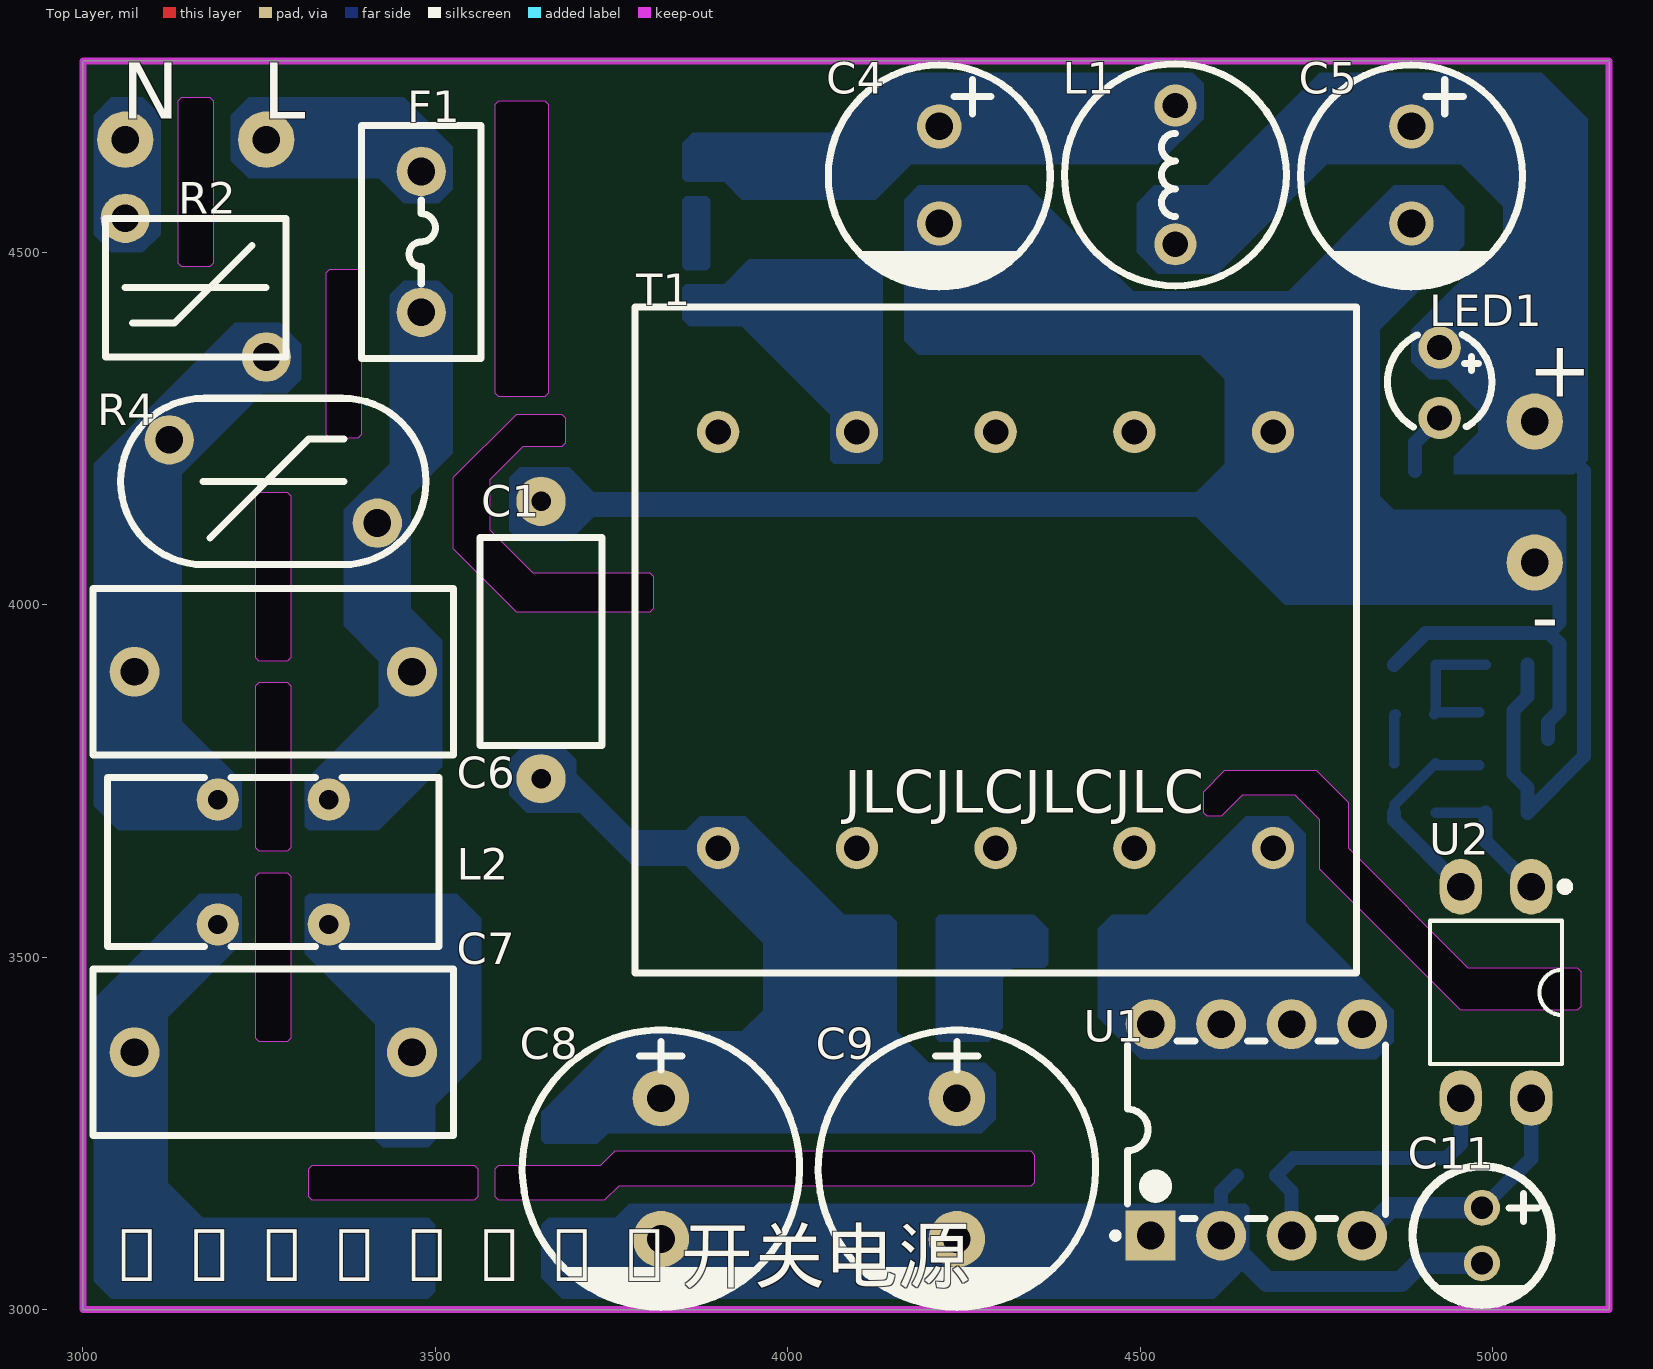
[diagram p0: Top Layer view]
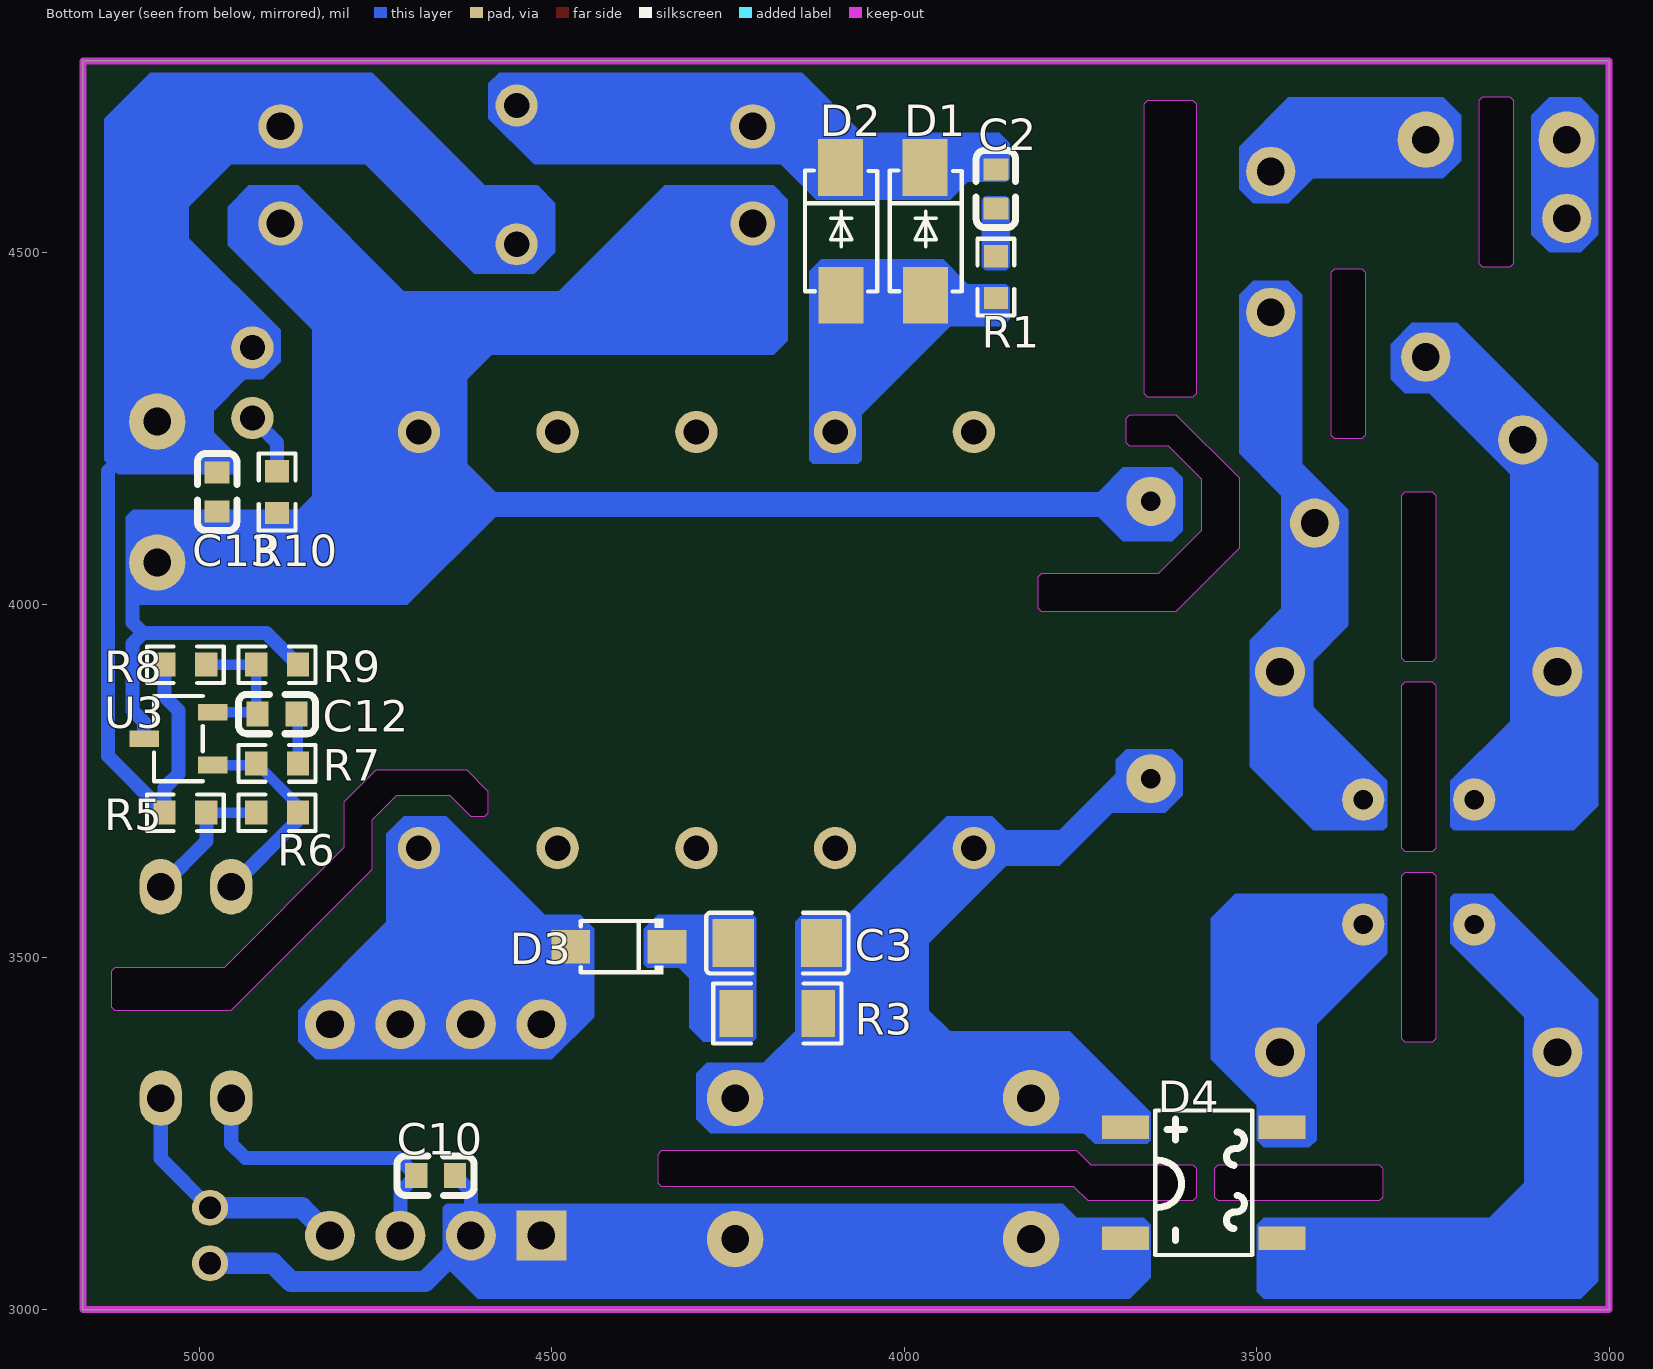
[diagram p1: Bottom Layer view, seen from below]
# Altium PCB MISC51479.pcbdoc
Units mil, origin at the board's own origin, x right, y up, seen from the top; angles counter-clockwise.
Board outline 2165.35 x 1771.65 mil, 2 copper layers (Top Layer, Bottom Layer), stack 62.206 mil thick; 35 components, 22 nets, 95 pads, 0 vias.

## Layer stack, top to bottom
Top Solder Mask Layer: solder mask 0.394, Dk 3.3
Top Layer: signal copper 1.379
Dielectric1: surface 59.449, FR4, Dk 4.5
Bottom Layer: signal copper 1.378
Bottom Solder Mask Layer: solder mask 0.394, Dk 3.3

## Board outline
3000,4771.65 3000,3000 5165.35,3000 5165.35,4771.65
cut-out: 3135,4715 3140,4720 3180,4720 3185,4715 3185,4485 3180,4480 3140,4480 3135,4485
cut-out: 3345,4471.26 3350,4476.26 3390,4476.26 3395,4471.26 3395,4241.26 3390,4236.26 3350,4236.26 3345,4241.26
cut-out: 3245,3885 3250,3890 3290,3890 3295,3885 3295,3655 3290,3650 3250,3650 3245,3655
cut-out: 3245,3615 3250,3620 3290,3620 3295,3615 3295,3385 3290,3380 3250,3380 3245,3385
cut-out: 3325,3155 3320,3160 3320,3200 3325,3205 3555,3205 3560,3200 3560,3160 3555,3155
cut-out: 3585,3200 3590,3205 3735,3205 3755,3225 4345,3225 4350,3220 4350,3180 4345,3175 3760,3175 3740,3155 3590,3155 3585,3160
cut-out: 3680,4225 3685,4230 3685,4265 3680,4270 3615,4270 3525,4180 3525,4080 3615,3990 3805,3990 3810,3995 3810,4040 3805,4045 3638.62,4045 3577.95,4105.67 3577.95,4177.95 3625,4225
cut-out: 3585,4710 3590,4715 3655,4715 3660,4710 3660,4300 3655,4295 3590,4295 3585,4300
cut-out: 4795,3720 4795,3655 4965,3485 5120,3485 5125,3480 5125,3430 5120,3425 4955,3425 4755,3625 4755,3695 4720,3730 4645,3730 4615,3700 4595,3700 4590,3705 4590,3735 4620,3765 4750,3765
cut-out: 3245,4155 3250,4160 3290,4160 3295,4155 3295,3925 3290,3920 3250,3920 3245,3925

## Design rules (kind name [scope] priority, off if disabled: settings)
BoardOutlineClearance copperThickness2oz_1 [All] p2 off: genericclearance=7.99 ignorepadtopadclearanceinfootprint=FALSE except(0: Arc-SplitContinuation Track-SplitContinuation SMDPad-SplitContinuation THPad-SplitContinuation Via-SplitContinuation Fill-SplitContinuation Region-SplitContinuation Poly-SplitContinuation Text-SplitContinuation Hole-SplitContinuation; 5.98: Arc-CutoutEdge Track-CutoutEdge SMDPad-CutoutEdge THPad-CutoutEdge Via-CutoutEdge Text-CutoutEdge; 6.9: Hole-OutlineEdge Hole-CutoutEdge; 10: Poly-OutlineEdge Poly-CutoutEdge; 11.81: Arc-OutlineEdge Track-OutlineEdge SMDPad-OutlineEdge THPad-OutlineEdge Via-OutlineEdge Fill-OutlineEdge Region-OutlineEdge Text-OutlineEdge Fill-CutoutEdge Region-CutoutEdge)
BoardOutlineClearance Plane_innerPlane_1 [All] p4 off: genericclearance=4.02 ignorepadtopadclearanceinfootprint=FALSE except(0: Arc-SplitContinuation Track-SplitContinuation SMDPad-SplitContinuation THPad-SplitContinuation Via-SplitContinuation Fill-SplitContinuation Region-SplitContinuation Poly-SplitContinuation Text-SplitContinuation Hole-SplitContinuation; 5.98: Arc-CutoutEdge Track-CutoutEdge SMDPad-CutoutEdge THPad-CutoutEdge Via-CutoutEdge Text-CutoutEdge; 6.9: Hole-OutlineEdge Hole-CutoutEdge; 10: Poly-OutlineEdge Poly-CutoutEdge; 11.81: Arc-OutlineEdge Track-OutlineEdge SMDPad-OutlineEdge THPad-OutlineEdge Via-OutlineEdge Fill-OutlineEdge Region-OutlineEdge Text-OutlineEdge Fill-CutoutEdge Region-CutoutEdge)
BoardOutlineClearance Copper_copperRegion_1 [All] p6 off: genericclearance=4.02 ignorepadtopadclearanceinfootprint=FALSE except(0: Arc-SplitContinuation Track-SplitContinuation SMDPad-SplitContinuation THPad-SplitContinuation Via-SplitContinuation Fill-SplitContinuation Region-SplitContinuation Poly-SplitContinuation Text-SplitContinuation Hole-SplitContinuation; 5.98: Arc-CutoutEdge Track-CutoutEdge SMDPad-CutoutEdge THPad-CutoutEdge Via-CutoutEdge Text-CutoutEdge; 6.9: Hole-OutlineEdge Hole-CutoutEdge; 10: Poly-OutlineEdge Poly-CutoutEdge; 11.81: Arc-OutlineEdge Track-OutlineEdge SMDPad-OutlineEdge THPad-OutlineEdge Via-OutlineEdge Fill-OutlineEdge Region-OutlineEdge Text-OutlineEdge Fill-CutoutEdge Region-CutoutEdge)
BoardOutlineClearance copperThickness1oz_1 [All] p8: genericclearance=4.02 ignorepadtopadclearanceinfootprint=FALSE except(0: Arc-SplitContinuation Track-SplitContinuation SMDPad-SplitContinuation THPad-SplitContinuation Via-SplitContinuation Fill-SplitContinuation Region-SplitContinuation Poly-SplitContinuation Text-SplitContinuation Hole-SplitContinuation; 5.98: Arc-CutoutEdge Track-CutoutEdge SMDPad-CutoutEdge THPad-CutoutEdge Via-CutoutEdge Text-CutoutEdge; 6.9: Hole-OutlineEdge Hole-CutoutEdge; 10: Poly-OutlineEdge Poly-CutoutEdge; 11.81: Arc-OutlineEdge Track-OutlineEdge SMDPad-OutlineEdge THPad-OutlineEdge Via-OutlineEdge Fill-OutlineEdge Region-OutlineEdge Text-OutlineEdge Fill-CutoutEdge Region-CutoutEdge)
Clearance copperThickness2oz [All] p1 off: gap=7.99 ignorepadtopadclearanceinfootprint=FALSE except(5.98: SMDPad-Track SMDPad-SMDPad THPad-Track SMDPad-THPad THPad-THPad Track-Via SMDPad-Via THPad-Via Via-Via Fill-SMDPad Region-SMDPad Fill-THPad Region-THPad Fill-Via Region-Via Fill-Fill Fill-Region Region-Region Arc-Track Arc-SMDPad Arc-THPad Arc-Via Fill-Arc Region-Arc Arc-Arc Text-Track SMDPad-Text Text-THPad Text-Via Fill-Text Region-Text Arc-Text Text-Text; 6.9: Hole-Track Hole-SMDPad Hole-THPad Hole-Via Fill-Hole Region-Hole Hole-Arc Hole-Text; 10: Poly-Track Poly-SMDPad Poly-THPad Poly-Via Poly-Fill Poly-Region Poly-Poly Poly-Arc Poly-Text Poly-Hole; 11.81: Fill-Track Region-Track)
Clearance Plane_innerPlane [All] p3 off: gap=4.02 ignorepadtopadclearanceinfootprint=FALSE except(5.98: SMDPad-Track SMDPad-SMDPad THPad-Track SMDPad-THPad THPad-THPad Track-Via SMDPad-Via THPad-Via Via-Via Fill-SMDPad Region-SMDPad Fill-THPad Region-THPad Fill-Via Region-Via Fill-Fill Fill-Region Region-Region Arc-Track Arc-SMDPad Arc-THPad Arc-Via Fill-Arc Region-Arc Arc-Arc Text-Track SMDPad-Text Text-THPad Text-Via Fill-Text Region-Text Arc-Text Text-Text; 6.9: Hole-Track Hole-SMDPad Hole-THPad Hole-Via Fill-Hole Region-Hole Hole-Arc Hole-Text; 10: Poly-Track Poly-SMDPad Poly-THPad Poly-Via Poly-Fill Poly-Region Poly-Poly Poly-Arc Poly-Text Poly-Hole; 11.81: Fill-Track Region-Track)
Clearance Copper_copperRegion [All] p5 off: gap=4.02 ignorepadtopadclearanceinfootprint=FALSE except(5.98: SMDPad-Track SMDPad-SMDPad THPad-Track SMDPad-THPad THPad-THPad Track-Via SMDPad-Via THPad-Via Via-Via Fill-SMDPad Region-SMDPad Fill-THPad Region-THPad Fill-Via Region-Via Fill-Fill Fill-Region Region-Region Arc-Track Arc-SMDPad Arc-THPad Arc-Via Fill-Arc Region-Arc Arc-Arc Text-Track SMDPad-Text Text-THPad Text-Via Fill-Text Region-Text Arc-Text Text-Text; 6.9: Hole-Track Hole-SMDPad Hole-THPad Hole-Via Fill-Hole Region-Hole Hole-Arc Hole-Text; 10: Poly-Track Poly-SMDPad Poly-THPad Poly-Via Poly-Fill Poly-Region Poly-Poly Poly-Arc Poly-Text Poly-Hole; 11.81: Fill-Track Region-Track)
Clearance copperThickness1oz [All] p7: gap=4.02 ignorepadtopadclearanceinfootprint=FALSE except(5.98: SMDPad-Track SMDPad-SMDPad THPad-Track SMDPad-THPad THPad-THPad Track-Via SMDPad-Via THPad-Via Via-Via Fill-SMDPad Region-SMDPad Fill-THPad Region-THPad Fill-Via Region-Via Fill-Fill Fill-Region Region-Region Arc-Track Arc-SMDPad Arc-THPad Arc-Via Fill-Arc Region-Arc Arc-Arc Text-Track SMDPad-Text Text-THPad Text-Via Fill-Text Region-Text Arc-Text Text-Text; 6.9: Hole-Track Hole-SMDPad Hole-THPad Hole-Via Fill-Hole Region-Hole Hole-Arc Hole-Text; 10: Poly-Track Poly-SMDPad Poly-THPad Poly-Via Poly-Fill Poly-Region Poly-Poly Poly-Arc Poly-Text Poly-Hole; 11.81: Fill-Track Region-Track)
DiffPairsRouting differentialPair [All] p1: maxlimit=6 minlimit=6 mostfreqgap=6 toplayer_minwidth=5 toplayer_prefwidth=10 toplayer_maxwidth=100 toplayer_mingap=6 toplayer_prefgap=6 toplayer_maxgap=6 bottomlayer_minwidth=5 bottomlayer_prefwidth=10 bottomlayer_maxwidth=100 bottomlayer_mingap=6 bottomlayer_prefgap=6 bottomlayer_maxgap=6 maxuncoupledlength=10
HoleToHoleClearance otherClearance [All] p1: gap=11.81 allowstackedmicrovias=TRUE
Length netLength [All] p1: minlimit=0 maxlimit=0
PasteMaskExpansion pasteMaskExpansion [All] p1: expansion=0
PlaneConnect innerPlane [All] p1: planeconnectstyle=Relief reliefexpansion=20 reliefentries=4 reliefconductorwidth=10 reliefairgap=10
PolygonConnect copperRegion [All] p1: connectstyle=Relief reliefconductorwidth=10 reliefentries=4 polygonreliefangle="90 Angle" airgapwidth=10 via.connectstyle=Relief via.reliefconductorwidth=10 via.reliefentries=4 via.polygonreliefangle="90 Angle" via.airgapwidth=10
RoutingVias viaSize [All] p1: holewidth=12.01 width=24.02 viastyle="Through Hole" minholewidth=11.81 minwidth=19.68 maxholewidth=248.03 maxwidth=393.7
SolderMaskExpansion solderMaskExpansion [IsVia] p1: expansion=-1000 istentingtop=TRUE
SolderMaskExpansion solderMaskExpansion [All] p2: expansion=2 istentingtop=FALSE
Width copperThickness2oz_2 [All] p1 off: maxlimit=100 minlimit=8 preferedwidth=10
Width copperThickness1oz_2 [All] p2: maxlimit=100 minlimit=5 preferedwidth=10

## Components (designator, comment, footprint, x,y, rotation, side; value= is the part's Value field where it differs from the comment)
C1 "1nF" CAP-TH_L7.5-W4.5-P10.00-D0.6 3650,3950 r90 top
C2 "100nF" C0603 3870,4590 r90 bottom
C3 "10nF" C1206 4180,3520 r180 bottom
C4 "470uF" CAP-TH_BD8.0-P3.50-D0.6-FD 4215,4610 r270 top
C5 "470uF" CAP-TH_BD8.0-P3.50-D0.6-FD 4885,4610 r270 top
C6 "100nF" CAP-TH_L13.0-W6.0-P10.00-D0.6 3270,3905 r0 top
C7 "100nF" CAP-TH_L13.0-W6.0-P10.00-D0.6 3270,3365 r0 top
C8 "22uF" CAP-TH_BD10.0-P5.00-D1.0-FD 3820,3200 r270 top
C9 "22uF" CAP-TH_BD10.0-P5.00-D1.0-FD 4240,3200 r270 top
C10 "1nF" C0603 4665,3190 r0 bottom
C11 "47uF" CAP-TH_BD5.0-P2.00-D0.8-FD 4985,3105 r270 top
C12 "100nF" C0603 4890,3845 r180 bottom
C13 "100nF" C0603 4975,4160 r90 bottom
D1 "SS310" SMA_L4.3-W2.6-LS5.0-FD 3970,4530 r90 bottom
D2 "SS310" SMA_L4.3-W2.6-LS5.0-FD 4090,4530 r90 bottom
D3 "FR107W" SOD-123FL_L2.7-W1.8-LS3.8-RD 4405,3515 r0 bottom
D4 "ABS210" ABF_L5.1-W4.4-P4.00-LS6.2-BL 3575,3180 r90 bottom
F1 "MST 2.5A 250V" FUSE-TH_L8.4-W4.3-P5.08-D1.0 3480,4515 r270 top
L1 "10uH" IND-TH_BD8.0-P5.00-D0.7 4550,4610 r270 top
L2 "PDMCAT953-102MLN" IND-TH_4P-L12.0-W6.0_PDMCAT953-501MLN 3270,3635 r180 top
LED1 "XL-302UGD" LED-TH_BD3.8-P2.54-FD_GREEN 4925,4315 r270 top
R1 "10K" R0603 3870,4465 r90 bottom
R2 "NTC33D-7" RES-TH_L6.5-W5.0-P5.00-D0.6-S4.40 3160,4450 r0 top
R3 "100K" R1206 4180,3420 r180 bottom
R4 "10D471K" RES-TH_L11.0-W6.0-P7.50-D0.8-S3.00 3270,4175 r180 top
R5 "1.5K" R0603 5020,3705 r0 bottom
R6 "1.5K" R0603 4890,3705 r0 bottom
R7 "10K" R0603 4890,3775 r180 bottom
R8 "20K" R0603 5020,3915 r0 bottom
R9 "2.2K" R0603 4890,3915 r0 bottom
R10 "4.7K" R0603 4890,4160 r90 bottom
T1 "" "EE25 5+5" 4295,3950 r90 top
U1 "DK125" DIP-8_L9.2-W6.4-P2.54-LS7.6-BL 4665,3255 r0 top
U2 "PC817C" DIP-4_L4.6-W6.5-P2.54-LS7.6-BL 5005,3450 r180 top
U3 "TL431AIDBZR" SOT-23-3_L2.9-W1.6-P1.90-LS2.8-BR 5030,3810 r180 bottom

## Footprints (in the part's own frame and the unit in brackets; to place one, negate y for a bottom-side part, rotate by r counter-clockwise, add the part's x,y. Pads: shape width x height; smd on the part's side, far side on the other; paste and mask are expansions set on the pad)
ABF_L5.1-W4.4-P4.00-LS6.2-BL [mm]
  rect 0.84x1.695 smd: 1(-2,-2.823) 2(2,-2.823) 3(2,2.822) 4(-2,2.822)
  silkscreen extent -2.6,-1.75 2.6,1.75
C0603 [mm]
  rect 0.8x0.9 smd: 1(-0.7,0) 2(0.7,0)
  silkscreen extent -1.39,-0.71 1.39,0.71
C1206 [mm]
  rect 1.485x1.728 smd paste-100 mask+0.051: 1(-1.593,0) 2(1.593,0)
  silkscreen extent -2.56,-1.09 2.56,1.09
CAP-TH_BD5.0-P2.00-D0.8-FD [mm]
  round 1.3 hole 0.8: 1(-1,0) 2(1,0)
  silkscreen extent -2.5,-2.5 2.5,2.5
CAP-TH_BD8.0-P3.50-D0.6-FD [mm]
  round 1.6 hole 1: 1(-1.75,0) 2(1.75,0)
  silkscreen extent -3.96,-4 4.04,4
CAP-TH_BD10.0-P5.00-D1.0-FD [mil]
  round 80 hole 39.37: 1(-100,0) 2(100,0)
  silkscreen extent -197,-197 200,197
CAP-TH_L7.5-W4.5-P10.00-D0.6 [mil]
  round 70 hole 27.56: 1(-196.85,0) 2(196.85,0)
  silkscreen extent -150,-87 146,87
CAP-TH_L13.0-W6.0-P10.00-D0.6 [mm]
  round 1.8 hole 1: 1(-5,0) 2(5,0)
  silkscreen extent -6.5,-3 6.5,3
DIP-4_L4.6-W6.5-P2.54-LS7.6-BL [mm]
  oval 1.524x2 hole 1: 1(-1.27,-3.81) 2(1.27,-3.81) 3(1.27,3.81) 4(-1.27,3.81)
  silkscreen extent -2.63,-3.96 2.38,2.58
DIP-8_L9.2-W6.4-P2.54-LS7.6-BL [mm]
  rect 1.8x1.8 hole 1: 1(-3.81,-3.81)
  round 1.8 hole 1: 2(-1.27,-3.81) 3(1.27,-3.81) 4(3.81,-3.81) 5(3.81,3.81) 6(1.27,3.81) 7(-1.27,3.81) 8(-3.81,3.81)
  silkscreen extent -5.18,-3.91 4.65,3.2
"EE25 5+5" [mil]
  round 60 hole 36: 1(-295.28,393.7) 2(-295.28,196.85) 3(-295.28,0) 4(-295.28,-196.85) 5(-295.28,-393.7) 6(295.28,-393.7) 7(295.28,-196.85) 8(295.28,0) 9(295.28,196.85) 10(295.28,393.7)
  silkscreen extent -472,-512 472,512
FUSE-TH_L8.4-W4.3-P5.08-D1.0 [mil]
  round 70 hole 39.37: 1(-100,0) 2(100,0)
  silkscreen extent -165,-85 165,85
IND-TH_4P-L12.0-W6.0_PDMCAT953-501MLN [mil]
  round 60 hole 27.56: 1(-78.74,-88.58) 2(-78.74,88.58) 3(78.74,88.58) 4(78.74,-88.58)
  silkscreen extent -235,-120 235,120
IND-TH_BD8.0-P5.00-D0.7 [mm]
  round 1.52 hole 0.91: 1(-2.5,0) 2(2.5,0)
  silkscreen extent -4,-4 4,4
LED-TH_BD3.8-P2.54-FD_GREEN [mil]
  round 60 hole 35.43: 1(-50,0) 2(50,0)
  silkscreen extent -68,-74 63,74
R0603 [mil]
  rect 31.75x34.02 smd paste-3937.01 mask+2: 1(-29.66,0) 2(29.66,0)
  silkscreen extent -55,-26 55,26
R1206 [mil]
  rect 47.54x66.97 smd paste-3937.01 mask+2: 1(-58.22,0) 2(58.22,0)
  silkscreen extent -91,-42 91,42
RES-TH_L6.5-W5.0-P5.00-D0.6-S4.40 [mil]
  round 70 hole 39.37: 1(-100,98.43) 2(100,-98.42)
  silkscreen extent -128,-98 128,98
RES-TH_L11.0-W6.0-P7.50-D0.8-S3.00 [mil]
  round 70 hole 39.37: 1(-147.64,59.06)
  round 70 hole 39.37 copper offset 0.01,-0.01: 2(147.63,-59.05)
  silkscreen extent -217,-118 217,118
SMA_L4.3-W2.6-LS5.0-FD [mm]
  rect 2.046x1.62 smd: 1(-2.304,-0.009) 2(2.304,0.009)
  silkscreen extent -2.17,-1.32 2.19,1.29
SOD-123FL_L2.7-W1.8-LS3.8-RD [mm]
  rect 1.4x1.2 smd: 1(-1.735,0) 2(1.735,0)
  silkscreen extent -1.6,-1 1.38,1
SOT-23-3_L2.9-W1.6-P1.90-LS2.8-BR [mm]
  rect 1.07x0.6 smd: 1(1.235,-0.95) 2(1.235,0.95) 3(-1.235,0)
  silkscreen extent -0.88,-1.54 0.88,1.54

## Free pads (board coordinates)
  round 80 hole 39.4: 1(3060,4660) 1(5060,4260) 2(3260,4660) 2(5060,4060)

## Nets (pads, with @x,y where several pads share a name; then routed paths per layer and width w, separated by ;. In a path a pad name is that pad's centre, name@x,y a point inside that pad or via, vN(x,y) a via of type N, cw(c..) or ccw(c..) an arc to the next point about the centre after c; other vN are vias at no path point)
$C1_1: C1.1 C3.2 C8.1 C9.1 D4.3 R3.2 T1.1
$C2_1: C2.1 R1.2
$C2_2: C2.2 C4.1 D1.2 D2.2 L1.1
$C3_1: C3.1 D3.1 R3.1
$C6_1: C6.1 L2.4 R2.2 R4.2
$C6_2: C6.2 F1.2 L2.1 R4.1
$C7_1: C7.1 D4.1 L2.3
$C7_2: C7.2 D4.2 L2.2
$C10_1: C8.2 C9.2 C10.1 C11.2 D4.4 U1.1 U1.2 | length 501.8
  Bottom Layer w20: U1.2 4615,3167.56 C10.1
  Bottom Layer w30: U1.2 4680,3040 4870,3040 4895.63,3065.63 C11.2
$C10_2: C10.2 U1.3 U2.3 | length 440.4
  Bottom Layer w20: U1.3 4715,3167.56 C10.2 4717.56,3215 4935,3215 4955,3235 U2.3
$C11_1: C11.1 U1.4 U2.4 | length 370.9
  Bottom Layer w20: C11.1 5055,3214.37 U2.4
  Bottom Layer w30: U1.4 4854.37,3144.37 C11.1
$C12_1: C12.1 R8.1 R9.2 U3.2 | length 203.4
  Bottom Layer w15: C12.1 C12.1@4919.66,3847.1 ; U3.2 4919.96,3847.4 C12.1@4919.66,3847.1 ; R8.1 R9.2 C12.1@4919.66,3847.1
$C12_2: C12.2 R7.2 | length 70.9
  Bottom Layer w15: R7.2 4860.34,3842.9 C12.2
$D1_1: D1.1 D2.1 R1.1 T1.9
$D3_2: D3.2 T1.5 U1.5 U1.6 U1.7 U1.8
$LED1_2: LED1.2 R10.2 | length 89.8
  Bottom Layer w20: R10.2 4890,4230 LED1.2
$R5_1: R5.1 R6.2 U2.1 | length 202.5
  Bottom Layer w15: R6.2 R5.1
  Bottom Layer w20: R5.1 4990.34,3664.66 U2.1
$R6_1: R6.1 R7.1 U2.2 U3.1 | length 301.5
  Bottom Layer w15: R6.1 4860.34,3715.68 R7.1 4922.06,3772.6 U3.1
  Bottom Layer w20: R6.1 4860.34,3694.66 U2.2
+24V: C5.1 C13.2 L1.2 LED1.1 pad.1@5060,4260 R5.2 R8.2 | length 843.6
  Bottom Layer w20: R8.2 5049.66,3869.66 5030,3850 5030,3760 5049.66,3740.34 R5.2 5130,3785.34 5130,4190 pad.1@5060,4260
GND: C1.2 C4.2 C5.2 C13.1 pad.2@5060,4060 R9.1 R10.1 T1.6 U3.3 | length 522
  Bottom Layer w20: R9.1 4905.34,3960 5080,3960 ; pad.2@5060,4060 5095,4025 5095,3975 5080,3960 ; U3.3 5078.62,3833.62 5095,3850 5095,3945 5080,3960
L: F1.1 pad.2@3260,4660
N: pad.1@3060,4660 R2.1
pads on no net: T1.2 T1.3 T1.4 T1.7 T1.8 T1.10

## Keep-outs
Board Outline Layer:
  region: 3135,4715 3140,4720 3180,4720 3185,4715 3185,4485 3180,4480 3140,4480 3135,4485
  region: 3135,4715 3140,4720 3180,4720 3185,4715 3185,4485 3180,4480 3140,4480 3135,4485
  region: 3345,4471.26 3350,4476.26 3390,4476.26 3395,4471.26 3395,4241.26 3390,4236.26 3350,4236.26 3345,4241.26
  region: 3345,4471.26 3350,4476.26 3390,4476.26 3395,4471.26 3395,4241.26 3390,4236.26 3350,4236.26 3345,4241.26
  region: 3245,3885 3250,3890 3290,3890 3295,3885 3295,3655 3290,3650 3250,3650 3245,3655
  region: 3245,3885 3250,3890 3290,3890 3295,3885 3295,3655 3290,3650 3250,3650 3245,3655
  region: 3245,3615 3250,3620 3290,3620 3295,3615 3295,3385 3290,3380 3250,3380 3245,3385
  region: 3245,3615 3250,3620 3290,3620 3295,3615 3295,3385 3290,3380 3250,3380 3245,3385
  region: 3325,3155 3320,3160 3320,3200 3325,3205 3555,3205 3560,3200 3560,3160 3555,3155
  region: 3325,3155 3320,3160 3320,3200 3325,3205 3555,3205 3560,3200 3560,3160 3555,3155
  region: 3585,3200 3590,3205 3735,3205 3755,3225 4345,3225 4350,3220 4350,3180 4345,3175 3760,3175 3740,3155 3590,3155 3585,3160
  region: 3585,3200 3590,3205 3735,3205 3755,3225 4345,3225 4350,3220 4350,3180 4345,3175 3760,3175 3740,3155 3590,3155 3585,3160
  region: 3680,4225 3685,4230 3685,4265 3680,4270 3615,4270 3525,4180 3525,4080 3615,3990 3805,3990 3810,3995 3810,4040 3805,4045 3638.62,4045 3577.95,4105.67 3577.95,4177.95 3625,4225
  region: 3680,4225 3685,4230 3685,4265 3680,4270 3615,4270 3525,4180 3525,4080 3615,3990 3805,3990 3810,3995 3810,4040 3805,4045 3638.62,4045 3577.95,4105.67 3577.95,4177.95 3625,4225
  region: 3585,4710 3590,4715 3655,4715 3660,4710 3660,4300 3655,4295 3590,4295 3585,4300
  region: 3585,4710 3590,4715 3655,4715 3660,4710 3660,4300 3655,4295 3590,4295 3585,4300
  region: 4795,3720 4795,3655 4965,3485 5120,3485 5125,3480 5125,3430 5120,3425 4955,3425 4755,3625 4755,3695 4720,3730 4645,3730 4615,3700 4595,3700 4590,3705 4590,3735 4620,3765 4750,3765
  region: 4795,3720 4795,3655 4965,3485 5120,3485 5125,3480 5125,3430 5120,3425 4955,3425 4755,3625 4755,3695 4720,3730 4645,3730 4615,3700 4595,3700 4590,3705 4590,3735 4620,3765 4750,3765
  region: 3245,4155 3250,4160 3290,4160 3295,4155 3295,3925 3290,3920 3250,3920 3245,3925
  region: 3245,4155 3250,4160 3290,4160 3295,4155 3295,3925 3290,3920 3250,3920 3245,3925
  lines w0.1: 3135,4485 3140,4480 3180,4480 3185,4485 3185,4715 3180,4720 3140,4720 3135,4715 3135,4485 ; 3245,3385 3250,3380 3290,3380 3295,3385 3295,3615 3290,3620 3250,3620 3245,3615 3245,3385 ; 3245,3655 3250,3650 3290,3650 3295,3655 3295,3885 3290,3890 3250,3890 3245,3885 3245,3655 ; 3245,3925 3250,3920 3290,3920 3295,3925 3295,4155 3290,4160 3250,4160 3245,4155 3245,3925 ; 3320,3160 3325,3155 3555,3155 3560,3160 3560,3200 3555,3205 3325,3205 3320,3200 3320,3160 ; 3345,4241.26 3350,4236.26 3390,4236.26 3395,4241.26 3395,4471.26 3390,4476.26 3350,4476.26 3345,4471.26 3345,4241.26 ; 3525,4080 3525,4180 3615,4270 3680,4270 3685,4265 3685,4230 3680,4225 3625,4225 3577.95,4177.95 3577.95,4105.67 3638.62,4045 3805,4045 3810,4040 3810,3995 3805,3990 3615,3990 3525,4080 ; 3585,3160 3590,3155 3740,3155 3760,3175 4345,3175 4350,3180 4350,3220 4345,3225 3755,3225 3735,3205 3590,3205 3585,3200 3585,3160 ; 3585,4300 3590,4295 3655,4295 3660,4300 3660,4710 3655,4715 3590,4715 3585,4710 3585,4300 ; 4590,3705 4595,3700 4615,3700 4645,3730 4720,3730 4755,3695 4755,3625 4955,3425 5120,3425 5125,3430 5125,3480 5120,3485 4965,3485 4795,3655 4795,3720 4750,3765 4620,3765 4590,3735 4590,3705
  lines w10: 3000,3000 3000,4771.65 5165.35,4771.65 5165.35,3000 3000,3000

## Other copper
Bottom Layer:
  region net $C2_1: 3855,4475 3885,4475 3890,4480 3890,4575 3885,4580 3855,4580 3850,4575 3850,4480
  region net $C10_1: 3650,3120 3660,3130 3755,3130 3775,3150 4650,3150 4655,3145 4655,3065 4605,3015 3680,3015 3650,3045
  region net $C1_1: 3780,3680 3855,3680 3875,3700 3940,3700 4080,3560 4145,3560 4155,3550 4155,3395 4200,3350 4280,3350 4295,3335 4295,3270 4275,3250 3745,3250 3730,3235 3655,3235 3650,3240 3650,3280 3765,3395 3935,3395 3965,3425 3965,3520 3855,3630 3780,3630 3705,3705 3630,3705 3605,3730 3605,3780 3620,3795 3685,3795 3700,3780 3700,3760
  region net GND: 3605,4180 3620,4195 3690,4195 3725,4160 4580,4160 4620,4200 4620,4320 4585,4355 4185,4355 4165,4375 4165,4575 4185,4595 4340,4595 4490,4445 4710,4445 4860,4595 4930,4595 4960,4565 4960,4510 4840,4390 4840,4155 4860,4135 5095,4135 5105,4125 5105,4010 5095,4000 4705,4000 4580,4125 3725,4125 3690,4090 3620,4090 3605,4105
  region net +24V: 4945,4185 4945,4210 4980,4245 4980,4275 4935,4320 4910,4320 4885,4345 4885,4390 5015,4520 5015,4565 4955,4625 4765,4625 4610,4470 4525,4470 4495,4500 4495,4570 4520,4595 4595,4595 4755,4755 5070,4755 5135,4690 5135,4205 5115,4185
  region net N: 3110,4695 3085,4720 3040,4720 3015,4695 3015,4525 3040,4500 3085,4500 3110,4525
  region net $C6_2: 3420,3920 3370,3970 3370,4135 3435,4200 3435,4440 3455,4460 3505,4460 3525,4440 3525,4215 3465,4155 3465,3995 3510,3950 3510,3770 3420,3680 3320,3680 3315,3685 3315,3750 3420,3855
  region net $C6_1: 3015,4200 3215,4400 3280,4400 3310,4370 3310,4320 3290,4300 3255,4300 3140,4185 3140,3835 3225,3750 3225,3685 3220,3680 3050,3680 3015,3715
  region net $C7_1: 3220,3590 3225,3585 3225,3520 3120,3415 3120,3180 3170,3130 3490,3130 3500,3120 3500,3025 3490,3015 3040,3015 3015,3040 3015,3440 3165,3590
  region net $C7_2: 3490,3230 3500,3240 3500,3290 3565,3355 3565,3555 3530,3590 3320,3590 3315,3585 3315,3505 3415,3405 3415,3240 3425,3230
  region net $C3_1: 4285,3380 4215,3380 4210,3385 4210,3555 4215,3560 4350,3560 4370,3540 4370,3490 4365,3485 4320,3485 4305,3470 4305,3400
  region net $D3_2: 4735,3675 4710,3700 4650,3700 4510,3560 4460,3560 4440,3540 4440,3415 4500,3355 4835,3355 4860,3380 4860,3425 4735,3550
  region net L: 3210,4695 3235,4720 3455,4720 3525,4650 3525,4590 3505,4570 3455,4570 3420,4605 3235,4605 3210,4630
  region net $D1_1: 3850,4450 3855,4455 3910,4455 3945,4490 4118,4490 4135,4473 4135,4205 4130,4200 4065,4200 4060,4205 4060,4270 3935,4395 3860,4395 3850,4405
  region net $C2_2: 3854.94,4600.06 3909.94,4600.06 3935,4575 4125,4575 4175,4625 4525,4625 4590,4690 4590,4740 4575,4755 4145,4755 4060,4670 3865,4670 3850,4655 3850,4605

## Silkscreen, mask and mechanical layers (free items; w line width, h text height)
Top Silkscreen Layer:
  text "N" at 3055,4690 h80
  text "L" at 3255,4690 h80
  text "+" at 5050,4295 h80
  text "-" at 5055,3945 h80
  text "JLCJLCJLCJLC" at 4080,3705 h60
  text "24V/0.8A开关电源" at 3025,3040 h75
Mechanical Layer:
  lines w0.1: 3135,4485 3140,4480 3180,4480 3185,4485 3185,4715 3180,4720 3140,4720 3135,4715 3135,4485 ; 3245,3385 3250,3380 3290,3380 3295,3385 3295,3615 3290,3620 3250,3620 3245,3615 3245,3385 ; 3245,3655 3250,3650 3290,3650 3295,3655 3295,3885 3290,3890 3250,3890 3245,3885 3245,3655 ; 3245,3925 3250,3920 3290,3920 3295,3925 3295,4155 3290,4160 3250,4160 3245,4155 3245,3925 ; 3320,3160 3325,3155 3555,3155 3560,3160 3560,3200 3555,3205 3325,3205 3320,3200 3320,3160 ; 3345,4241.26 3350,4236.26 3390,4236.26 3395,4241.26 3395,4471.26 3390,4476.26 3350,4476.26 3345,4471.26 3345,4241.26 ; 3525,4080 3525,4180 3615,4270 3680,4270 3685,4265 3685,4230 3680,4225 3625,4225 3577.95,4177.95 3577.95,4105.67 3638.62,4045 3805,4045 3810,4040 3810,3995 3805,3990 3615,3990 3525,4080 ; 3585,3160 3590,3155 3740,3155 3760,3175 4345,3175 4350,3180 4350,3220 4345,3225 3755,3225 3735,3205 3590,3205 3585,3200 3585,3160 ; 3585,4300 3590,4295 3655,4295 3660,4300 3660,4710 3655,4715 3590,4715 3585,4710 3585,4300 ; 4590,3705 4595,3700 4615,3700 4645,3730 4720,3730 4755,3695 4755,3625 4955,3425 5120,3425 5125,3430 5125,3480 5120,3485 4965,3485 4795,3655 4795,3720 4750,3765 4620,3765 4590,3735 4590,3705